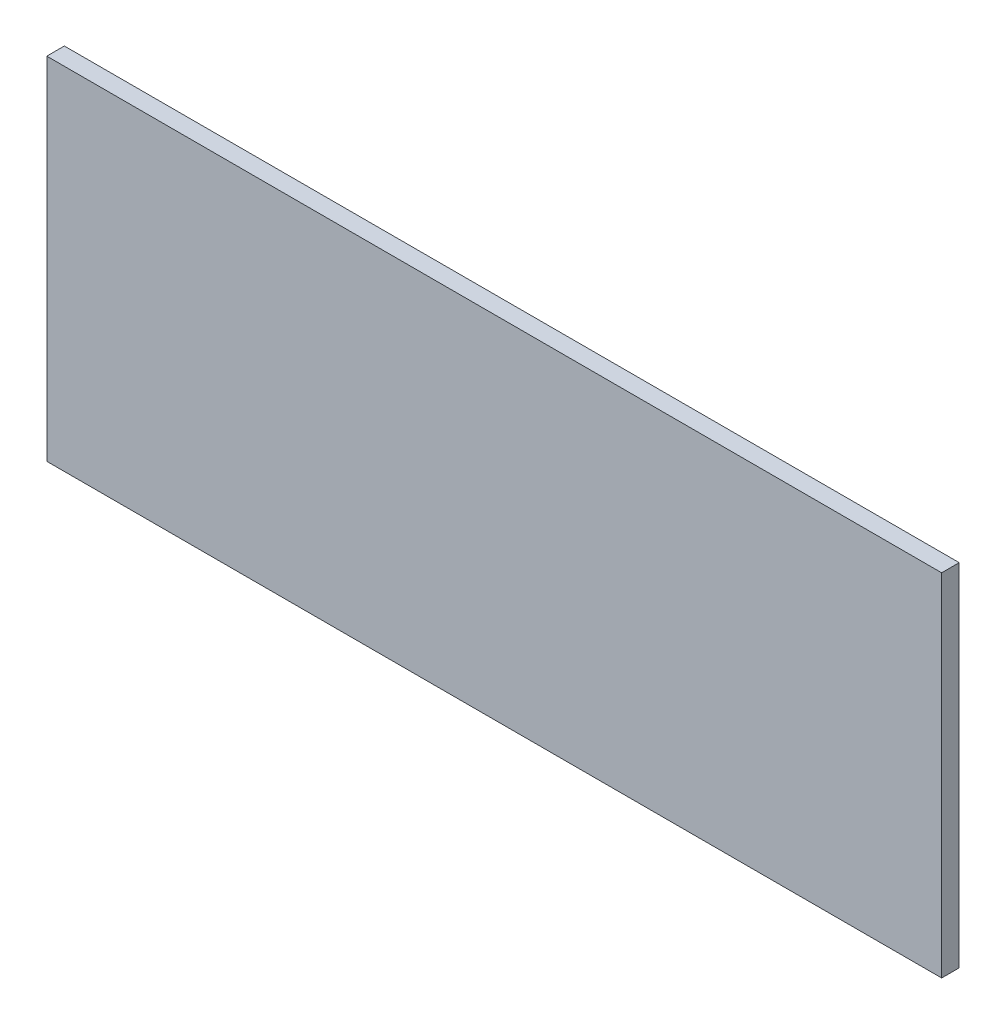
SolidWorks part; units mm, degrees
ref_plane "前视基准面" through (0, 0, 0) normal (0, 0, 1) x (1, 0, 0)
ref_plane "上视基准面" through (0, 0, 0) normal (0, 1, 0) x (1, 0, 0)
ref_plane "右视基准面" through (0, 0, 0) normal (1, 0, 0) x (0, 0, -1)
sketch "草图2" plane through (0, 0, 0) normal (0, 0, 1) x (1, 0, 0)
  line L0 (0, 0) -> (255, 0)
  line L1 (255, 0) -> (255, 100)
  line L2 (255, 100) -> (0, 100)
  line L3 (0, 100) -> (0, 0)
extrude "凸台-拉伸1" add sketch "草图2" against normal blind 5
sketch "草图3" plane through (0, 0, 0) normal (0, 0, 1) x (1, 0, 0)
  line L0 (0, 100) -> (10, 100)
  line L1 (255, 100) -> (0, 100) construction
  line L2 (0, 100) -> (0, 90)
  line L3 (0, 100) -> (0, 0) construction
  line L4 (0, 90) -> (10, 100)
  line L5 (255, 100) -> (245, 100)
  line L6 (255, 100) -> (255, 90)
  line L7 (255, 0) -> (255, 100) construction
  line L8 (255, 90) -> (245, 100)
  line L9 (255, 0) -> (255, 10)
  line L10 (0, 0) -> (0, 10)
  line L11 (0, 0) -> (10, 0)
  line L12 (255, 0) -> (245, 0)
  line L13 (0, 0) -> (255, 0) construction
  line L14 (255, 10) -> (245, 0)
  line L15 (10, 0) -> (0, 10)
extrude "切除-拉伸1" cut sketch "草图3" against normal blind 5
sketch "草图4" plane through (0, 0, -5) normal (0, 0, -1) x (-1, 0, 0)
  line L0 (-242, 16.5) -> (-215, 16.5)
  line L2 (-13, 83.5) -> (-40, 83.5)
  line L4 (-215, 96.5) -> (-242, 96.5)
  line L5 (-215, 3.5) -> (-242, 3.5)
  line L6 (-242, 83.5) -> (-215, 83.5)
  line L7 (-127.5, 100) -> (-127.5, 0)
  line L8 (-245, 100) -> (-10, 100) construction
  line L9 (-10, 0) -> (-245, 0) construction
  line L10 (-40, 3.5) -> (-13, 3.5)
  line L11 (-40, 96.5) -> (-13, 96.5)
  line L12 (-13, 16.5) -> (-40, 16.5)
  arc A0 (-242, 16.5) -> (-242, 3.5) centre (-242, 10) ccw
  arc A1 (-215, 3.5) -> (-215, 16.5) centre (-215, 10) ccw
  arc A2 (-215, 96.5) -> (-215, 83.5) centre (-215, 90) cw
  arc A3 (-242, 83.5) -> (-242, 96.5) centre (-242, 90) cw
  arc A4 (-13, 83.5) -> (-13, 96.5) centre (-13, 90) ccw
  arc A5 (-40, 96.5) -> (-40, 83.5) centre (-40, 90) ccw
  arc A6 (-40, 3.5) -> (-40, 16.5) centre (-40, 10) cw
  arc A7 (-13, 16.5) -> (-13, 3.5) centre (-13, 10) cw
extrude "切除-拉伸2" cut sketch "草图4" against normal blind 21 contours A3 L6 A2 L4 | L11 A5 L2 A4 | A7 L12 A6 L10 | L5 A1 L0 A0
sketch "草图5" plane through (0, 0, -5) normal (0, 0, -1) x (-1, 0, 0)
  line L0 (-255, 90) -> (-255, 100)
  line L1 (-255, 10) -> (-255, 90) construction
  line L2 (-255, 100) -> (0, 100)
  line L3 (0, 100) -> (0, 0)
  line L4 (0, 0) -> (-255, 0)
  line L5 (-255, 0) -> (-255, 90)
extrude "凸台-拉伸2" add sketch "草图5" against normal blind 5
